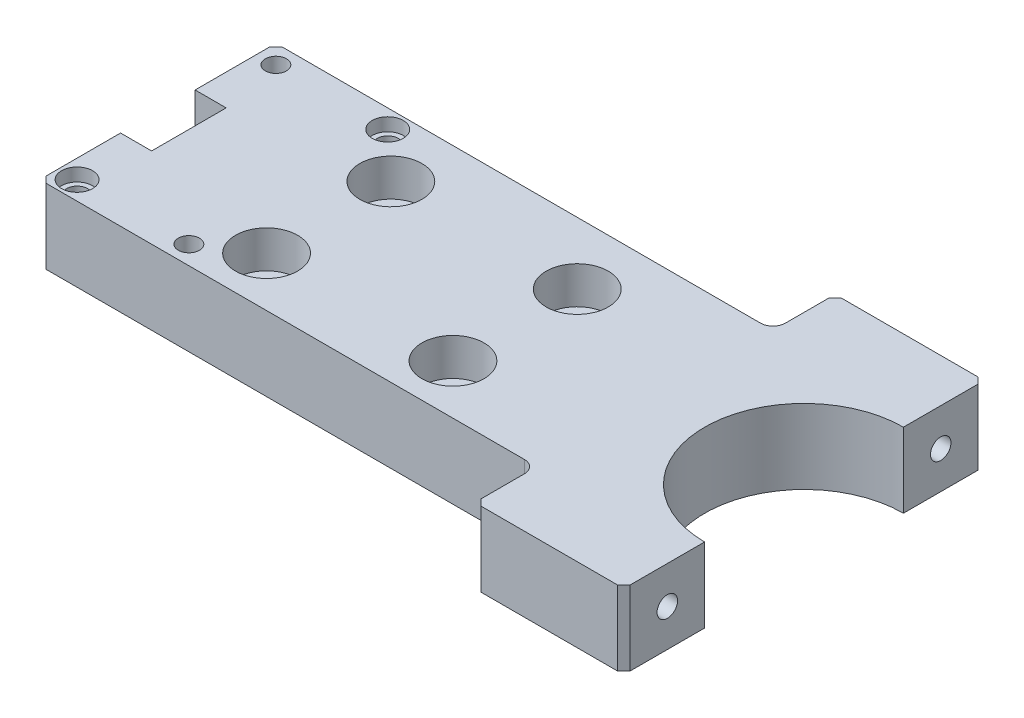
SolidWorks part; units mm, degrees
material "45"
ref_plane "Front Plane" through (0, 0, 0) normal (0, 0, 1) x (1, 0, 0)
ref_plane "Top Plane" through (0, 0, 0) normal (0, 1, 0) x (1, 0, 0)
ref_plane "Right Plane" through (0, 0, 0) normal (1, 0, 0) x (0, 0, -1)
sketch "Sketch1" plane through (0, 0, 0) normal (0, 0, 1) x (1, 0, 0)
  line L1 (0, 0) -> (104, 0)
  line L2 (0, 0) -> (0, 12)
  line L3 (0, 12) -> (104, 12)
  line L4 (104, 0) -> (104, 12)
  dimension "D1" = 12
  dimension "D2" = 104
extrude "Boss-Extrude1" add sketch "Sketch1" along normal blind 38
sketch "Sketch2" plane through (0, 12, 0) normal (0, 1, 0) x (1, 0, 0)
  line L0 (0, -38) -> (0, 0) construction
  line L1 (0, -13) -> (5, -13)
  line L2 (0, -13) -> (0, -25)
  line L3 (0, -25) -> (5, -25)
  line L4 (5, -13) -> (5, -25)
  line L5 (104, -19) -> (0, -19) construction
  line L6 (104, -38) -> (104, 0) construction
  dimension "D1" = 12
  dimension "D2" = 5
extrude "Cut-Extrude1" cut sketch "Sketch2" against normal through all
sketch "Sketch3" plane through (0, 12, 0) normal (0, 1, 0) x (1, 0, 0)
  line L0 (104, -38) -> (104, 0) construction
  circle A0 centre (104, -19) radius 16
  dimension "D1" = 32
extrude "Cut-Extrude2" cut sketch "Sketch3" against normal through all
sketch "Sketch4" plane through (0, 0, 0) normal (0, 0, -1) x (-1, 0, 0)
  line L0 (0, 0) -> (-104, 0) construction
  line L1 (-104, 12) -> (-80, 12)
  line L2 (-104, 12) -> (-104, 0)
  line L3 (-104, 0) -> (-80, 0)
  line L4 (-80, 12) -> (-80, 0)
  dimension "D1" = 24
extrude "Boss-Extrude2" add sketch "Sketch4" along normal blind 10
sketch "Sketch5" plane through (0, 0, 38) normal (0, 0, 1) x (1, 0, 0)
  line L4 (104, 0) -> (104, 12)
  line L5 (80, 0) -> (104, 0)
  line L6 (80, 12) -> (80, 0)
  line L7 (104, 12) -> (80, 12)
  line L8 (104, 0) -> (104, 12)
  line L9 (80, 0) -> (104, 0)
  line L10 (80, 12) -> (80, 0)
  line L11 (104, 12) -> (80, 12)
  dimension "D1" = 0
extrude "Boss-Extrude3" add sketch "Sketch5" along normal blind 10
chamfer "Chamfer1" distance 1 angle 45 6 edges at (0, 6, 0) (0, 6, 38) (104, 6, 48) (80, 6, 48) (104, 6, -10) (80, 6, -10)
fillet "Fillet1" radius 2 2 edges
hole_wizard "Hole size per socket head cap screw type 1" positions "Sketch7" profile "Sketch6" counterbore size "M3" standard "Gb" end condition through all
sketch "Sketch7" plane through (0, 0, 0) normal (0, -1, 0) x (-1, 0, 0)
  circle A0 centre (-21, -3) radius 2.5 construction
  circle A1 centre (-3, -3) radius 1.2295 construction
  circle A2 centre (-3, -35) radius 2.5 construction
  circle A3 centre (-21, -35) radius 1.2295 construction
  point P0 (-3, -35)
  point P2 (-21, -3)
  point P6 (-3, -3)
  point P8 (-21, -35)
sketch "Sketch6" plane through (3, 0, 35) normal (1, 0, 0) x (0, 0, -1)
  line L0 (0, 0) -> (0, 12)
  line L1 (0, 12) -> (1.7, 12)
  line L3 (1.7, 12) -> (1.7, 4)
  line L4 (1.7, 4) -> (2.75, 4)
  line L5 (2.75, 4) -> (2.75, 0)
  line L7 (2.75, 0) -> (0, 0)
  line L11 (0, -6.35) -> (0, 107.95) construction
  dimension "通孔孔直径" = 3.4
  dimension "通孔孔深度" = 12
  dimension "柱形沉头孔直径" = 5.5
  dimension "柱形沉头孔深度" = 4
sketch "Sketch8" plane through (0, 12, 0) normal (0, 1, 0) x (1, 0, 0)
  circle A0 centre (3, -35) radius 2.5
  circle A1 centre (21, -3) radius 2.5
  dimension "D1" = 5
extrude "Cut-Extrude3" cut sketch "Sketch8" against normal blind 2.1
hole_wizard "Hole size per socket head cap screw type 2" positions "Sketch10" profile "Sketch9" counterbore size "M5" standard "Gb" end condition through all
sketch "Sketch10" plane through (0, 12, 0) normal (0, 1, 0) x (1, 0, 0)
  circle A4 centre (28.5, -30) radius 4.5 construction
  circle A5 centre (58.5, -30) radius 4.5 construction
  circle A6 centre (58.5, -10) radius 4.5 construction
  circle A7 centre (28.5, -10) radius 4.5 construction
  point P0 (28.5, -10)
  point P2 (28.5, -30)
  point P4 (58.5, -10)
  point P6 (58.5, -30)
sketch "Sketch9" plane through (28.5, 12, 10) normal (1, 0, 0) x (0, 0, 1)
  line L0 (0, 0) -> (0, 12)
  line L1 (0, 12) -> (2.75, 12)
  line L3 (2.75, 12) -> (2.75, 6)
  line L4 (2.75, 6) -> (5, 6)
  line L5 (5, 6) -> (5, 0)
  line L7 (5, 0) -> (0, 0)
  line L11 (0, -6.35) -> (0, 107.95) construction
  dimension "通孔孔直径" = 5.5
  dimension "通孔孔深度" = 12
  dimension "柱形沉头孔直径" = 10
  dimension "柱形沉头孔深度" = 6
sketch "Sketch11" plane through (0, 0, 0) normal (0, -1, 0) x (1, 0, 0)
  circle A0 centre (28.5, 30) radius 4.5
  circle A1 centre (58.5, 10) radius 4.5
  dimension "D1" = 9
extrude "Cut-Extrude4" cut sketch "Sketch11" against normal blind 2.1
hole_wizard "M4 Tapped Hole1" positions "Sketch13" profile "Sketch12" tap size "M4" standard "Iso"
sketch "Sketch13" plane through (104, 0, 0) normal (1, 0, 0) x (0, 0, -1)
  line L0 (-3, 6) -> (3, 6) construction
  line L1 (-3, 12) -> (-3, 0) construction
  line L3 (-35, 0) -> (-35, 12) construction
  line L4 (-35, 6) -> (-41, 6) construction
  point P0 (3, 6)
  point P2 (-41, 6)
  dimension "D1" = 44
sketch "Sketch12" plane through (104, 6, -3) normal (0, 1, 0) x (0, 0, -1)
  line L0 (0, 0) -> (0, 12.4914)
  line L1 (0, 12.4914) -> (1.65, 11.5)
  line L2 (1.65, 11.5) -> (1.65, 0)
  line L5 (1.65, 0) -> (0, 0)
  line L10 (0, 12.4914) -> (-1.65, 11.5) construction
  line L11 (0, -6.35) -> (0, 107.95) construction
  dimension "螺纹孔钻头直径" = 3.3
  dimension "螺纹孔钻头深度" = 11.5
  dimension "导头角度" = 118
cosmetic thread "Hole thread 1" parameters "D1"=8, "D2"=4
cosmetic thread "Hole thread 2" parameters "D1"=8, "D2"=4
